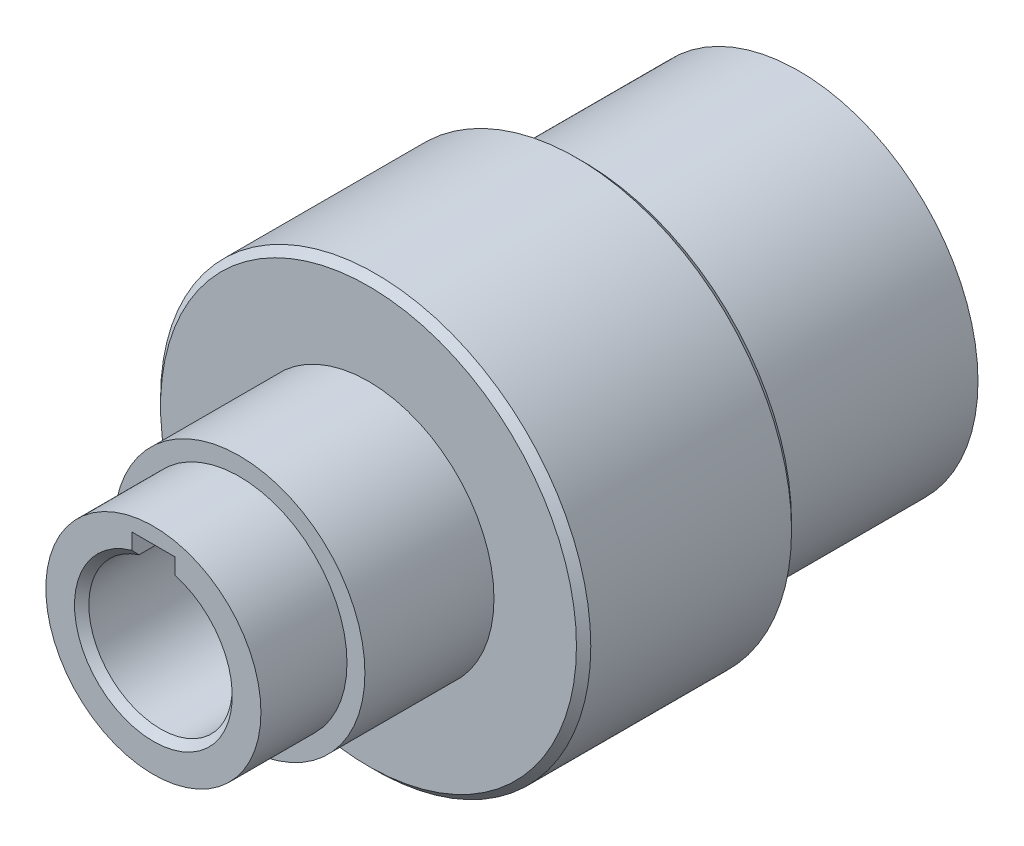
SolidWorks part; units mm, degrees
material "Q235A"
ref_plane "前视基准面" through (0, 0, 0) normal (0, 0, 1) x (1, 0, 0)
ref_plane "上视基准面" through (0, 0, 0) normal (0, 1, 0) x (1, 0, 0)
ref_plane "右视基准面" through (0, 0, 0) normal (1, 0, 0) x (0, 0, -1)
sketch "草图1" plane through (0, 0, 0) normal (0, 0, 1) x (1, 0, 0)
  circle A0 centre (0, 0) radius 25
  dimension "D1" = 50
extrude "凸台-拉伸1" add sketch "草图1" along normal blind 30
sketch "草图2" plane through (0, 0, 30) normal (0, 0, 1) x (1, 0, 0)
  circle A0 centre (0, 0) radius 30
  dimension "D1" = 60
extrude "凸台-拉伸2" add sketch "草图2" along normal blind 40
sketch "草图3" [suppressed] plane through (0, 0, 70) normal (0, 0, 1) x (1, 0, 0)
  circle A0 centre (0, 0) radius 15
  dimension "D1" = 30
sketch "草图4" plane through (0, 0, 0) normal (0, 0, -1) x (-1, 0, 0)
  circle A0 centre (0, 0) radius 10
  dimension "D1" = 20
extrude "切除-拉伸1" cut sketch "草图4" against normal through all
sketch "草图6" plane through (0, 0, 70) normal (0, 0, 1) x (1, 0, 0)
  line L0 (0, 30) -> (0, 0) construction
  line L1 (-13.0767, 27) -> (13.0767, 27)
  line L2 (27, 13.0767) -> (27, -13.0767)
  line L3 (13.0767, -27) -> (-13.0767, -27)
  line L4 (-27, -13.0767) -> (-27, 13.0767)
  line L5 (0, 0) -> (13.0767, 27) construction
  arc A0 (27, -13.0767) -> (27, 13.0767) centre (0, 0) ccw
  circle A1 centre (0, 0) radius 30
  arc A2 (13.0767, 27) -> (-13.0767, 27) centre (0, 0) ccw
  arc A3 (-13.0767, -27) -> (13.0767, -27) centre (0, 0) ccw
  arc A4 (-27, 13.0767) -> (-27, -13.0767) centre (0, 0) ccw
  dimension "D2" = 3
  dimension "D1" = 0
  dimension "D3" = 4
extrude "切除-拉伸2" [suppressed] cut sketch "草图6" against normal offset from surface (35 mm away) 5
sketch "草图11" plane through (0, 0, 70) normal (0, 0, 1) x (1, 0, 0)
  line L0 (0, 0) -> (0, 31.5305) construction
  line L2 (-3, 9.5394) -> (3, 9.5394)
  line L3 (-3, 9.5394) -> (-3, 12.8)
  line L4 (-3, 12.8) -> (3, 12.8)
  line L5 (3, 9.5394) -> (3, 12.8)
  line L6 (-3, 9.5394) -> (3, 12.8) construction
  line L7 (-3, 12.8) -> (3, 9.5394) construction
  circle A0 centre (0, 0) radius 10 construction
  point P3 (0, 11.1697)
  dimension "D1" = 6
  dimension "D2" = 2.8
extrude "切除-拉伸3" cut sketch "草图11" against normal through all
sketch "草图12" plane through (0, 0, 0) normal (0, 0, -1) x (-1, 0, 0)
  circle A0 centre (0, 0) radius 15
  dimension "D1" = 30
extrude "切除-拉伸4" cut sketch "草图12" against normal blind 30
sketch "草图13" plane through (0, 0, 70) normal (0, 0, 1) x (1, 0, 0)
  line L0 (3, 9.5394) -> (3, 12.8) construction
  line L1 (-3, 12.8) -> (-3, 9.5394) construction
  line L2 (3, 12.8) -> (-3, 12.8) construction
  line L3 (3, 9.5394) -> (3, 12.8)
  line L4 (-3, 12.8) -> (-3, 9.5394)
  line L5 (3, 12.8) -> (-3, 12.8)
  circle A0 centre (0, 0) radius 17.5
  arc A1 (-3, 9.5394) -> (3, 9.5394) centre (0, 0) ccw construction
  arc A2 (-3, 9.5394) -> (3, 9.5394) centre (0, 0) ccw
  dimension "D1" = 35
extrude "凸台-拉伸4" add sketch "草图13" along normal blind 20
sketch "草图14" plane through (0, 0, 70) normal (0, 0, 1) x (1, 0, 0)
  circle A0 centre (0, 0) radius 17.5 construction
  circle A1 centre (0, 0) radius 17.5
  circle A4 centre (0, 0) radius 30
  circle A8 centre (0, 0) radius 30
  dimension "D1" = 0
extrude "切除-拉伸5" cut sketch "草图14" against normal blind 10
hole_wizard "M8 螺纹孔1" positions "草图7" profile "草图8" tap size "M8" standard "ISO"
sketch "草图7" [suppressed] plane through (-27, 0, 0) normal (-1, 0, 0) x (0, 0, 1)
  line L0 (35, 0) -> (70, 0)
  line L1 (35, -13.0767) -> (35, 13.0767) construction
  line L4 (60, 13.0767) -> (60, -13.0767) construction
  point P0 (54, 0)
  dimension "D1" = 6
sketch "草图8" plane through (-27, 0, 54) normal (0, 1, 0) x (0, 0, 1)
  line L0 (0, 0) -> (0, 57)
  line L1 (0, 57) -> (3.4, 57)
  line L2 (3.4, 57) -> (3.4, 0)
  line L5 (3.4, 0) -> (0, 0)
  line L11 (0, -6.35) -> (0, 107.95) construction
  dimension "通孔螺纹孔钻头直径" = 6.8
  dimension "通孔螺纹孔钻头深度" = 57
cosmetic thread "孔螺蚊线1" [suppressed] parameters "D2"=8
hole_wizard "M8 螺纹孔2" positions "草图9" profile "草图10" tap size "M8" standard "ISO"
sketch "草图9" [suppressed] plane through (0, 27, 0) normal (0, 1, 0) x (1, 0, 0)
  line L0 (0, -35) -> (0, -70) construction
  line L1 (13.0767, -35) -> (-13.0767, -35) construction
  line L4 (13.0767, -60) -> (-13.0767, -60) construction
  point P0 (0, -54)
  dimension "D1" = 6
sketch "草图10" plane through (0, 27, 54) normal (1, 0, 0) x (0, 0, 1)
  line L0 (0, 0) -> (0, 57)
  line L1 (0, 57) -> (3.4, 57)
  line L2 (3.4, 57) -> (3.4, 0)
  line L5 (3.4, 0) -> (0, 0)
  line L11 (0, -6.35) -> (0, 107.95) construction
  dimension "通孔螺纹孔钻头直径" = 6.8
  dimension "通孔螺纹孔钻头深度" = 57
cosmetic thread "孔螺蚊线2" [suppressed] parameters "D2"=8
sketch "草图15" plane through (0, 0, 90) normal (0, 0, 1) x (1, 0, 0)
  circle A0 centre (0, 0) radius 15
  circle A1 centre (0, 0) radius 17.5
  circle A2 centre (0, 0) radius 17.5
  dimension "D2" = 30
  dimension "D1" = 0
extrude "切除-拉伸6" cut sketch "草图15" against normal blind 12
chamfer "倒角2" distance 1 angle 45 4 edges at (30, 0, 60) (30, 0, 30) (0, -10, 90) (-15, 0, 0)
